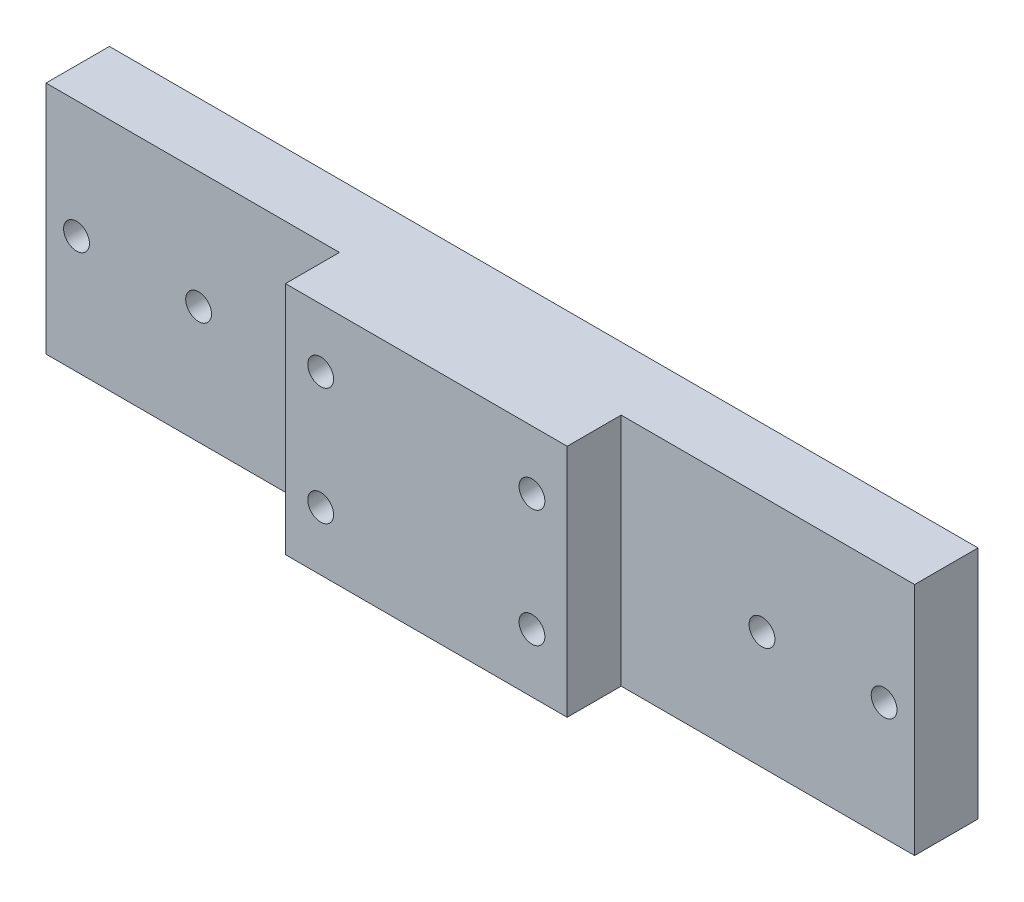
from build123d import *

# Parameters (mm, degrees)
SKETCH1_W                                         = 185
SKETCH1_H                                         = 50
BOSS_EXTRUDE1_DEPTH                               = 25
SKETCH2_W                                         = 62.5
SKETCH2_H                                         = 50
CUT_EXTRUDE1_DEPTH                                = 11.5
M5_SOCKET_HEAD_CAP_SCREW_COUNTERBORE1_D           = 5.5
M5_SOCKET_HEAD_CAP_SCREW_COUNTERBORE1_CBORE_D     = 10
M5_SOCKET_HEAD_CAP_SCREW_COUNTERBORE1_CBORE_DEPTH = 5.7
M5_SOCKET_HEAD_CAP_SCREW_COUNTERBORE2_D           = 5.5
M5_SOCKET_HEAD_CAP_SCREW_COUNTERBORE2_CBORE_D     = 10
M5_SOCKET_HEAD_CAP_SCREW_COUNTERBORE2_CBORE_DEPTH = 5.7


with BuildPart() as part:
    # Sketch1 → Boss-Extrude1 (new body)
    with BuildSketch(Plane.XY):
        Rectangle(SKETCH1_W, SKETCH1_H)
    extrude(amount=BOSS_EXTRUDE1_DEPTH)

    # Sketch2 → Cut-Extrude1 (cut)
    with BuildSketch(Plane.XY.offset(25)):
        with Locations((-61.25, 0)):
            Rectangle(SKETCH2_W, SKETCH2_H)
        with Locations((61.25, 0)):
            Rectangle(SKETCH2_W, SKETCH2_H)
    extrude(amount=-CUT_EXTRUDE1_DEPTH, mode=Mode.SUBTRACT)

    # M5 socket head cap screw counterbore1 (through all)
    with Locations(Plane(origin=(0, 0, 0), x_dir=(-1, 0, 0), z_dir=(0, 0, -1))):
        with Locations((-86, 0), (-60, 0), (60, 0), (86, 0)):
            CounterBoreHole(M5_SOCKET_HEAD_CAP_SCREW_COUNTERBORE1_D / 2, M5_SOCKET_HEAD_CAP_SCREW_COUNTERBORE1_CBORE_D / 2, M5_SOCKET_HEAD_CAP_SCREW_COUNTERBORE1_CBORE_DEPTH)

    # M5 socket head cap screw counterbore2 (through all)
    with Locations(Plane(origin=(0, 0, 0), x_dir=(-1, 0, 0), z_dir=(0, 0, -1))):
        with Locations((-22.5, 12.5), (-22.5, -12.5), (22.5, 12.5), (22.5, -12.5)):
            CounterBoreHole(M5_SOCKET_HEAD_CAP_SCREW_COUNTERBORE2_D / 2, M5_SOCKET_HEAD_CAP_SCREW_COUNTERBORE2_CBORE_D / 2, M5_SOCKET_HEAD_CAP_SCREW_COUNTERBORE2_CBORE_DEPTH)


solid = part.part
